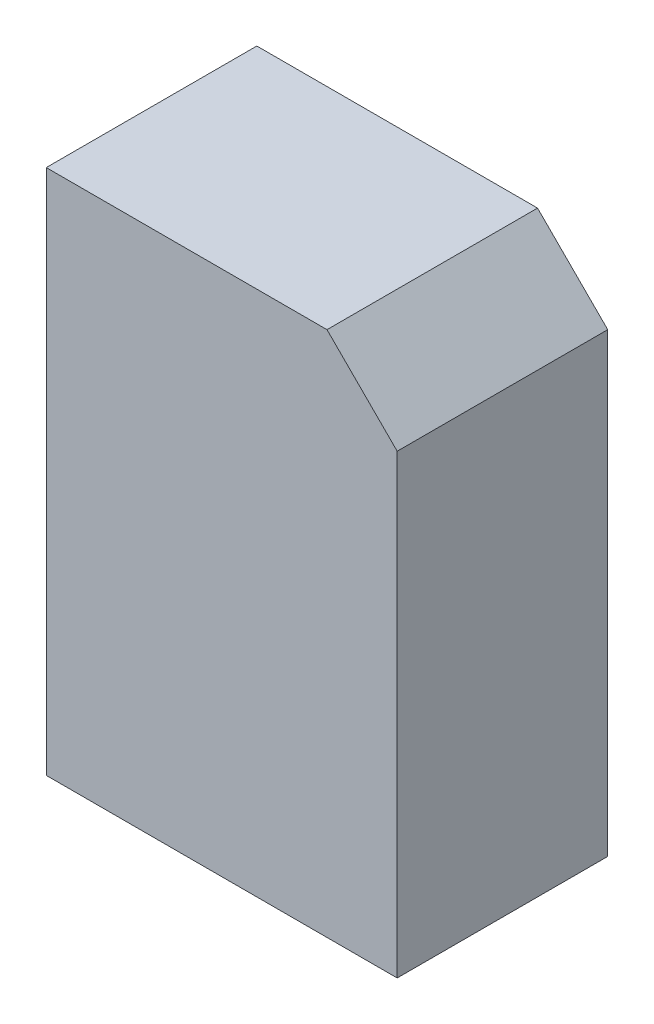
from build123d import *

# Parameters (mm, degrees)
SKETCH1_W           = 1000
SKETCH1_H           = 1500
BOSS_EXTRUDE1_DEPTH = 600
CHAMFER1_SIZE       = 200


with BuildPart() as part:
    # Sketch1 → Boss-Extrude1 (new body)
    with BuildSketch(Plane.XY):
        Rectangle(SKETCH1_W, SKETCH1_H)
    extrude(amount=BOSS_EXTRUDE1_DEPTH)

    # Chamfer1
    chamfer1_edges = [part.edges().sort_by_distance(p)[0] for p in [
        (500, 750, 300),
    ]]
    chamfer(chamfer1_edges, length=CHAMFER1_SIZE)


solid = part.part
